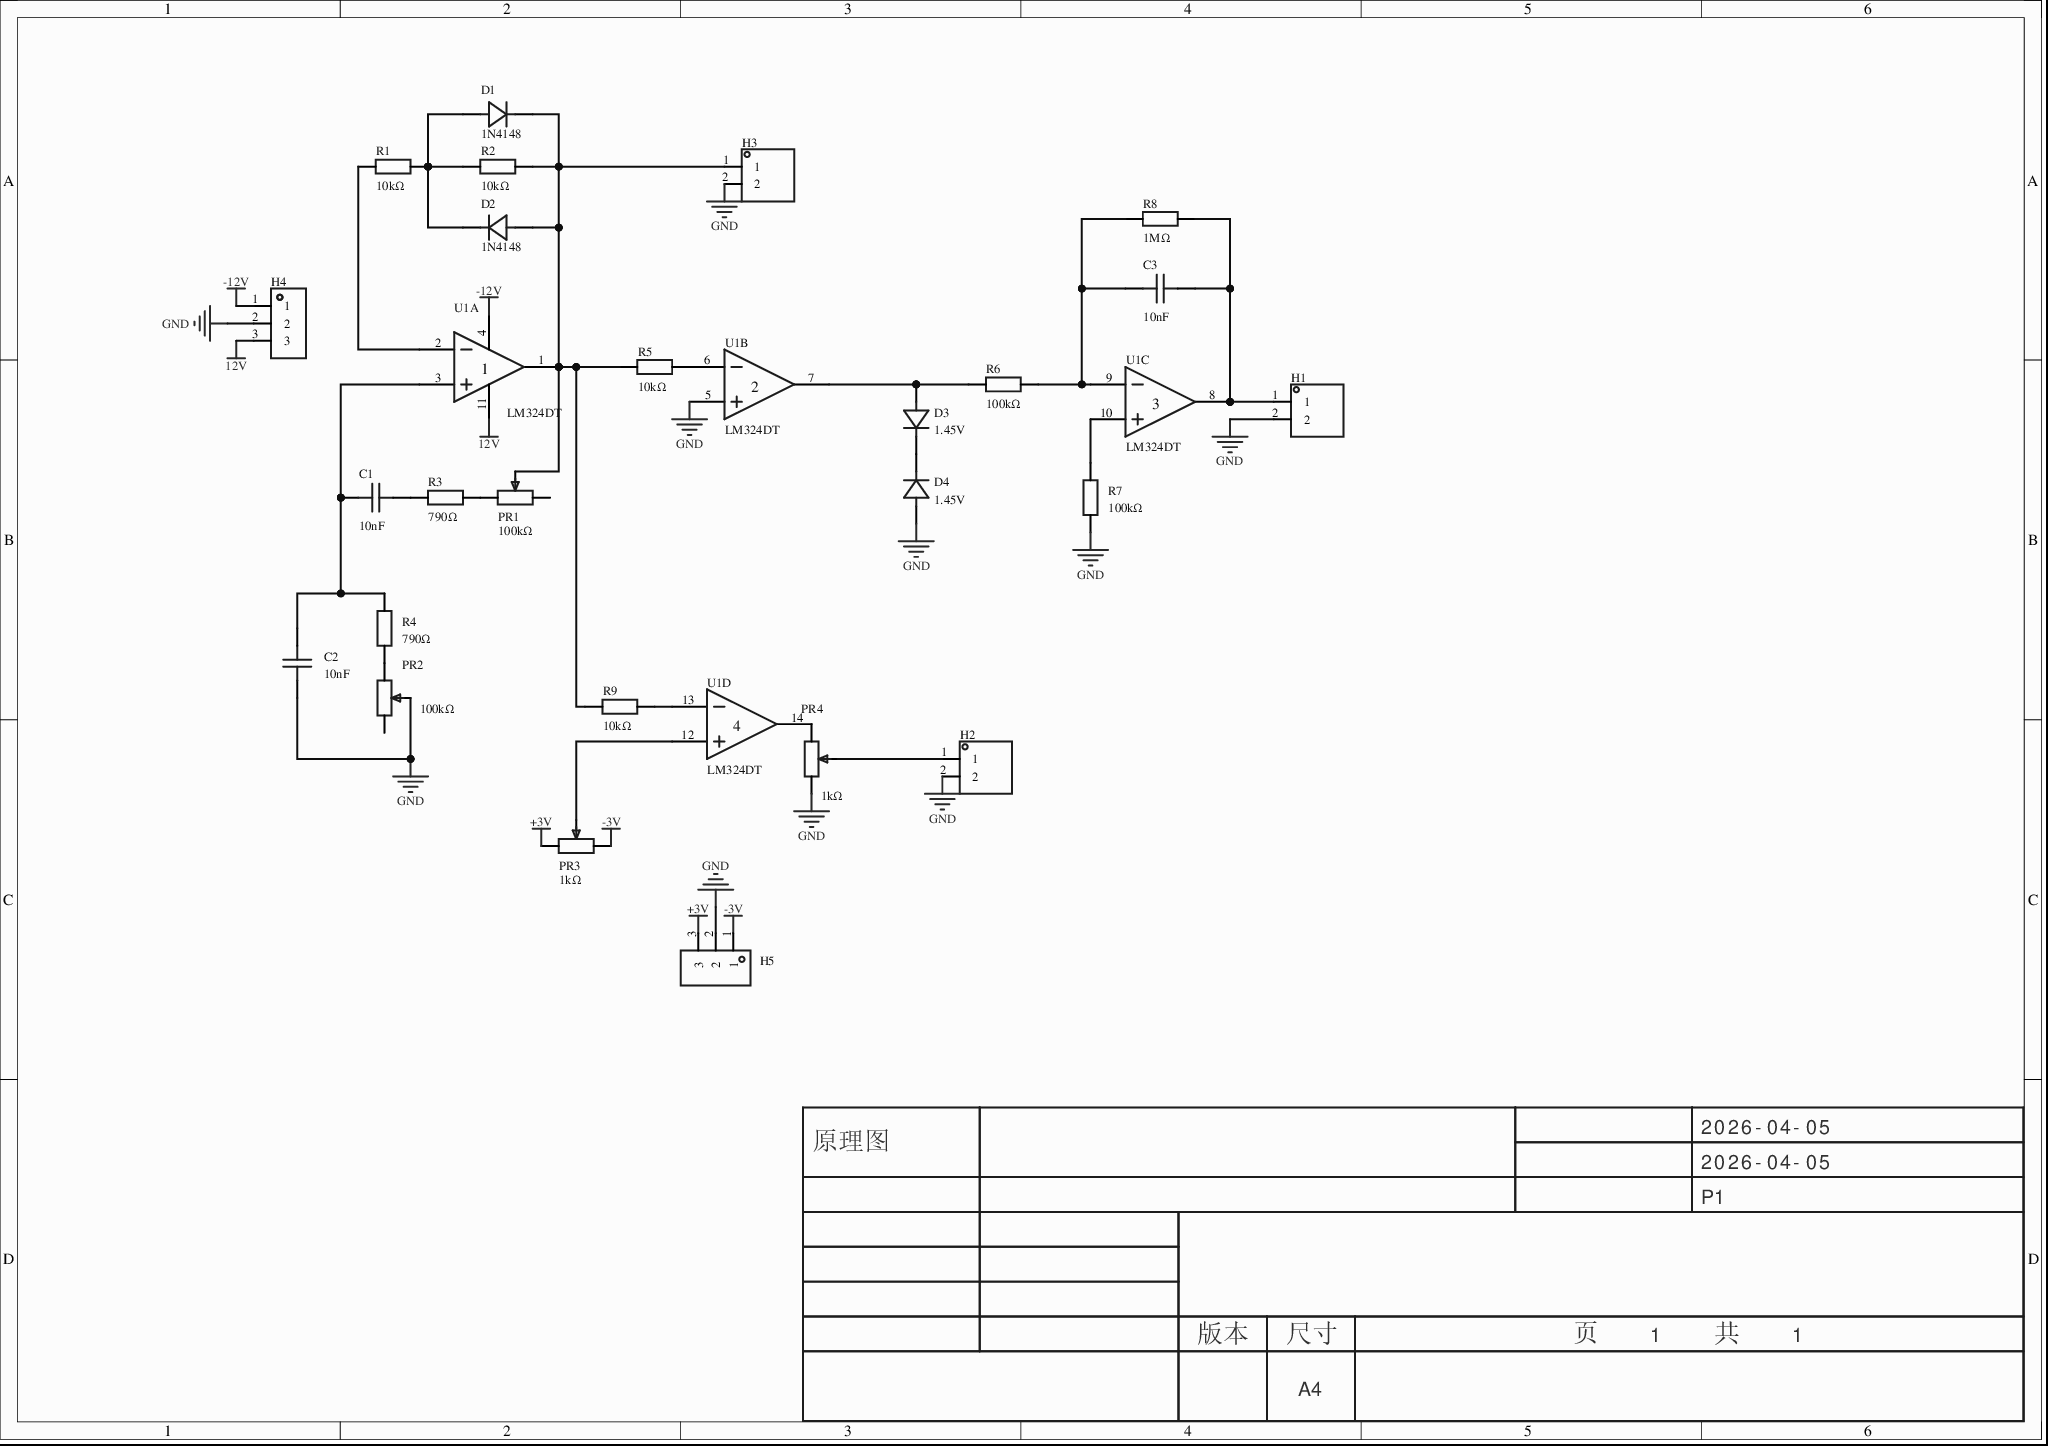
[diagram p0: MISC51375-3.schdoc]
# Altium project MISC51375-2.PrjPcb
1 sheet, 26 parts. Net scope: global (net labels, ports and power ports of the same name join across sheets).
Board file: MISC51375.pcbdoc

## Sheet MISC51375-3.schdoc
size 297 x 209 mm; Version: V1.0; @Project Name: MISC51375; @Update Date: 2026-04-05; @Create Date: 2026-04-05; @Board Name: MISC51375; @Create Time: 17:30:51; @Page Count: 1; @Page No: 1; @Schematic Name: MISC51375; @Update Time: 17:30:51; Size: A4

### Parts
C1  10nF  [CAP-TH_L7.2-W3.5-P5.00-D0.6]
C2  10nF  [CAP-TH_L7.2-W3.5-P5.00-D0.6]
C3  10nF  [CAP-TH_L7.2-W3.5-P5.00-D0.6]
D1  1N4148  [DO-35_BD2.2-L4.0-D0.50_1N4148]
D2  1N4148  [DO-35_BD2.2-L4.0-D0.50_1N4148]
D3  1.45V  [DO-35_BD2.0-L4.2-P8.20-D0.5-RD]
D4  1.45V  [DO-35_BD2.0-L4.2-P8.20-D0.5-RD]
H1  (no value)  [HDR-TH_2P-P2.54-V-M-1]
H2  (no value)  [HDR-TH_2P-P2.54-V-M-1]
H3  (no value)  [HDR-TH_2P-P2.54-V-M-1]
H4  (no value)  [HDR-TH_3P-P2.54-V-M]
H5  (no value)  [HDR-TH_3P-P2.54-V-M]
PR1  100kΩ  [R_3296]
PR2  100kΩ  [R_3296]
PR3  1kΩ  [R_3296]
PR4  1kΩ  [R_3296]
R1  10kΩ  [Res_1/8W]
R2  10kΩ  [Res_1/8W]
R3  790Ω  [Res_1/8W]
R4  790Ω  [Res_1/8W]
R5  10kΩ  [Res_1/8W]
R6  100kΩ  [Res_1/8W]
R7  100kΩ  [Res_1/8W]
R8  1MΩ  [Res_1/8W]
R9  10kΩ  [Res_1/8W]
U1  LM324DT  [DIP-14_L19.2-W6.6-P2.54-LS10.9-BL]  (parts A,B,C,D of 4)

### Nets
12V: H4.3 U1.11(VCC-)
+3V: H5.3 PR3.3
-3V: H5.1 PR3.1
-12V: H4.1 U1.4(VCC+)
GND: C2.1 D4.2(A) H1.2 H2.2 H3.2 H4.2 H5.2 PR2.2 PR4.1 R7.1 U1.5(IN2+)
NetC1_1: C1.1 C2.2 R4.1 U1.3(IN1+)
NetC1_2: C1.2 R3.1
NetC3_1: C3.1 R6.2 R8.1 U1.9(IN3-)
NetC3_2: C3.2 H1.1 R8.2 U1.8(OUT3)
NetD1_1: D1.1(A) D2.2(C) R1.2 R2.1
NetD1_2: D1.2(C) D2.1(A) H3.1 PR1.2 R2.2 R5.1 R9.1 U1.1(OUT1)
NetD3_1: D3.1(K) D4.1(K)
NetD3_2: D3.2(A) R6.1 U1.7(OUT2)
NetH2_1: H2.1 PR4.2
NetPR1_3: PR1.3 R3.2
NetPR2_3: PR2.3 R4.2
NetPR3_2: PR3.2 U1.12(IN4+)
NetPR4_3: PR4.3 U1.14(OUT4)
NetR1_1: R1.1 U1.2(IN1-)
NetR5_2: R5.2 U1.6(IN2-)
NetR7_2: R7.2 U1.10(IN3+)
NetR9_2: R9.2 U1.13(IN4-)

Not connected (* = marked no-connect by the designer): PR1 1; PR2 1

### Notes on the sheet
- 2026-04-05
- 原理图
- P1
- 版本
- 尺寸
- A4
- 页    1    共    1

### Library data of the parts
C1-C3 = BFC237051103: 容值:10nF;精度:±10%;额定电压:400V;介电材料:金属化聚酯;工作温度:-55℃~+105℃;; Manufacturer: VISHAY(威世); AddInBom: yes; ModelId: a68e1e188062432283baa1666d1dc16a0819f05c4eef4c71ace90d822a990e87; ModelTransform: 283.464,138.1887,0,0,0,0,0,0,-196.85; Tolerance: ±10%; Voltage Rated: 400V; Dielectric Material: 金属化聚酯; Symbol: BFC237051103; Device: BFC237051103; LCSC Part Name: 10nF ±10% 400V; SupplierPart: C3767808; ManufacturerPart: BFC237051103; Supplier Footprint: -; JLCPCB Part Class: Extended Part; Datasheet: https://atta.szlcsc.com/upload/public/pdf/source/20231215/C7F0606909F0C3498BE7598C12553344.pdf; Supplier: LCSC; ConvertToPcb: yes; FootprintName: CAP-TH_L7.2-W3.5-P5.00-D0.6; ModelName: CAP-TH_L7.2-W3.5-P5.00-D0.6; Value: 10nF; Operating Temperature: -55℃~+105℃
D1 D2 = 1N4148_C18195411: 正向压降(Vf):1V@10mA;直流反向耐压(Vr):100V;整流电流:150mA;反向恢复时间(Trr):4ns;; Manufacturer: LJ(朗捷); AddInBom: yes; ModelId: b29439ed7b924f62acded4384188502f0819f05c4eef4c71ace90d822a990e87; ModelTransform: 334.645,87.008,0,0,0,0,0,0,-196.85; Voltage - DC Reverse(Vr): 100V; Current - Rectified: 150mA; Pd - Power Dissipation: 500mW; Reverse Leakage Current (Ir): 5mA; Reverse Recovery Time (trr): 4ns; Operating Junction Temperature Range: -60℃~+200℃; Non-Repetitive Peak Forward Surge Current: 500mA; Symbol: 1N4148_C18195411; Device: 1N4148_C18195411; LCSC Part Name: 100V 150mA; SupplierPart: C18195411; ManufacturerPart: 1N4148; Supplier Footprint: DO-35; JLCPCB Part Class: Extended Part; Datasheet: https://item.szlcsc.com/datasheet/1N4148/19344798.html; Supplier: LCSC; ConvertToPcb: yes; FootprintName: DO-35_BD2.2-L4.0-D0.50_1N4148; ModelName: DO-35_BD2.2-L4.0-D0.50_1N4148; Voltage - Forward(Vf@If): 1V@10mA
D3 D4 = 1SS54: Manufacturer: RENESAS(瑞萨)/IDT; AddInBom: yes; ModelId: 6e6fa891745c42b796728c269d94cdcf0819f05c4eef4c71ace90d822a990e87; ModelName: DO-35_D1.9-L3.9-P8.2; ModelTransform: 342.519,74.82103,0,0,0,0,-0.197,1.181,-137.795; Symbol: 1SS54; Device: 1SS54; Manufacturer Part: 1.45V; LCSC Part Name: 1SS54; SupplierPart: C17462718; Supplier Footprint: DO-35; JLCPCB Part Class: Extended Part; Datasheet: https://item.szlcsc.com/datasheet/1SS54/18591911.html; Supplier: LCSC; ConvertToPcb: yes; FootprintName: DO-35_BD2.0-L4.2-P8.20-D0.5-RD
H1-H3 = HDR-M_2.54_1x2P: Symbol: 210S-1*2P L=11.6MMGold-plated black; ConvertToPcb: yes; ModelId: 79b2e9f2d70a4d68a1b7098f27c6d4c50819f05c4eef4c71ace90d822a990e87; ModelName: HDR-M-2.54_1x2; ModelTransform: 200,100,0,0,0,0,0,0,-118.11; Device: HDR-M_2.54_1x2P; AddInBom: yes; SupplierPart: C124375; Supplier Footprint: 插件; FootprintName: HDR-TH_2P-P2.54-V-M-1
H4 H5 = HDR-M_2.54_1x3P: AddInBom: yes; ModelId: bb473b6d38ff42a99216a4fcdbdcc4cb0819f05c4eef4c71ace90d822a990e87; ModelName: HDR-TH_3P-P2.54-M-LI-1X3P; ModelTransform: 300.03877,100,0,0,0,0,0,0,-118.11; Symbol: HDR-M_2.54_1x3P; Device: HDR-M_2.54_1x3P; ConvertToPcb: yes; FootprintName: HDR-TH_3P-P2.54-V-M; SupplierPart: C2937625; Supplier Footprint: 插件
PR1-PR4 = R_3296: ConvertToPcb: yes; ModelId: b182808559bb43bda9e7de64b64134cb0819f05c4eef4c71ace90d822a990e87; ModelName: 3296W; ModelTransform: 373.98,188.96,590.49,180,0,0,0,0,-140; Symbol: R_3296; Device: R_3296; AddInBom: yes; Supplier Footprint: 直插; FootprintName: R_3296
  PR1 PR2: Value: 100kΩ
  PR3 PR4: Value: 1kΩ
R1-R9 = Res_AXIAL-1/8W: Symbol: 电阻; ConvertToPcb: yes; ModelId: b2b5ae7ae4c642178fe0039925c86a3f0819f05c4eef4c71ace90d822a990e87; ModelName: RES-TH_BD1.8-L3.2-P7.20-D0.4; ModelTransform: 282.86,66.88,253.09,0,0,0,0,0,-191; Device: Res_AXIAL-1/8W; AddInBom: yes; Supplier Footprint: 轴向引线; FootprintName: Res_1/8W
  R1 R2 R5 R9: Value: 10kΩ
  R3 R4: Value: 790Ω
  R6 R7: Value: 100kΩ
  R8: Value: 1MΩ
U1 = LM324DT: 放大器数:4;轨到轨:-;增益带宽积(GBW):1.3MHz;输入失调电压(Vos):5mV;压摆率(SR):20V/us;输入偏置电流(Ib):300nA;; Manufacturer: ST(意法半导体); Relevance: []; AddInBom: yes; ModelId: 8dbf5b715d42428c85558507ae5a252b0819f05c4eef4c71ace90d822a990e87; ModelName: SOIC-14_L8.6-W3.9-H1.8-LS6.0-P1.27; ModelTransform: 338.583,236.22,0,0,0,0,0,0.001,0; Number of Channels: 4; Maximum Power Supply Range (Vdd-Vss): 30V; Gain Bandwidth Product: 1.3MHz; Vos - Input Offset Voltage: 5mV; Input Offset Voltage Drift(Vos TC): 30uV/℃; Slew Rate: 20V/us; Ib - Input Bias Current: 300nA; Input Offset Current(Ios): 20nA; Input Voltage Noise Density: 40nV/√Hz@1kHz; Common Mode Rejection Ratio(CMRR): 80dB; Input offset current drift(Ios TC): 200pA/℃; Quiescent Current: 1.2mA; Output Current: 70mA; Single supply: 3V~30V; Dual Supply: -15V~-1.5V；1.5V~15V; Symbol: LM324DT; Device: LM324DT; LCSC Part Name: 低功耗四路运算放大器; SupplierPart: C71035; ManufacturerPart: LM324DT; Supplier Footprint: SOIC-14; JLCPCB Part Class: Basic Part; Datasheet: https://item.szlcsc.com/datasheet/LM324DT/72134.html; Supplier: LCSC; ConvertToPcb: yes; FootprintName: DIP-14_L19.2-W6.6-P2.54-LS10.9-BL; Rail to Rail: -; Operating Temperature: 0℃~+70℃; Features: -